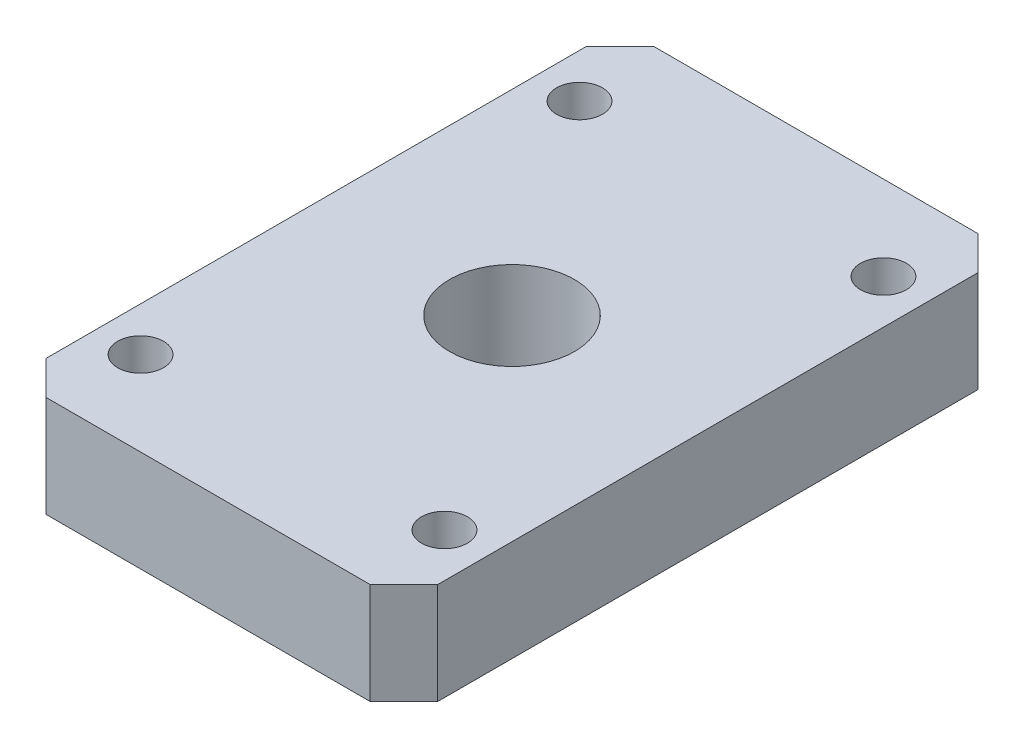
SolidWorks part; units mm, degrees
ref_plane "前视基准面" through (0, 0, 0) normal (0, 0, 1) x (1, 0, 0)
ref_plane "上视基准面" through (0, 0, 0) normal (0, 1, 0) x (1, 0, 0)
ref_plane "右视基准面" through (0, 0, 0) normal (1, 0, 0) x (0, 0, -1)
sketch "草图1" plane through (0, 0, 0) normal (0, 1, 0) x (1, 0, 0)
  line L1 (-29, 45) -> (29, 45)
  line L2 (-29, 45) -> (-29, -45)
  line L3 (-29, -45) -> (29, -45)
  line L4 (29, 45) -> (29, -45)
  line L5 (-29, 45) -> (29, -45) construction
  line L6 (-29, -45) -> (29, 45) construction
  point P0 (0, 0)
  dimension "D1" = 58
  dimension "D2" = 90
extrude "凸台-拉伸1" add sketch "草图1" along normal mid plane 15
hole_wizard "M8 螺纹孔1" positions "草图3" profile "草图2" tap size "M8" standard "ISO"
sketch "草图3" plane through (0, -7.5, 0) normal (0, 1, 0) x (1, 0, 0)
  line L0 (0, 0) -> (44.1668, 0) construction
  point P0 (-22.5, 32.5)
  point P2 (22.5, 32.5)
  point P16 (22.5, -32.5)
  point P17 (-22.5, -32.5)
  dimension "D1" = 32.5
  dimension "D2" = 22.5
  dimension "D3" = 45
cosmetic thread "孔螺蚊线6" parameters "D1"=16, "D2"=8
cosmetic thread "孔螺蚊线7" parameters "D1"=16, "D2"=8
cosmetic thread "孔螺蚊线8" parameters "D1"=16, "D2"=8
cosmetic thread "孔螺蚊线9" parameters "D1"=16, "D2"=8
sketch "草图2" plane through (-22.5, -7.5, -32.5) normal (1, 0, 0) x (0, 0, -1)
  line L0 (0, 0) -> (0, 21.7929)
  line L1 (0, 21.7929) -> (3.4, 19.75)
  line L2 (3.4, 19.75) -> (3.4, 0)
  line L5 (3.4, 0) -> (0, 0)
  line L10 (0, 21.7929) -> (-3.4, 19.75) construction
  line L11 (0, -6.35) -> (0, 107.95) construction
  dimension "螺纹孔钻头直径" = 6.8
  dimension "螺纹孔钻头深度" = 19.75
  dimension "导头角度" = 118
hole_wizard "M20x1.5 螺纹孔1" positions "草图5" profile "草图4" tap size "M20x1.5" standard "ISO"
sketch "草图5" plane through (0, 7.5, 0) normal (0, 1, 0) x (1, 0, 0)
  point P0 (0, 0)
cosmetic thread "孔螺蚊线5" parameters "D1"=16, "D2"=20
sketch "草图4" plane through (0, 7.5, 0) normal (1, 0, 0) x (0, 0, 1)
  line L0 (0, 0) -> (0, 50.058)
  line L1 (0, 50.058) -> (9.25, 44.5)
  line L2 (9.25, 44.5) -> (9.25, 0)
  line L5 (9.25, 0) -> (0, 0)
  line L10 (0, 50.058) -> (-9.25, 44.5) construction
  line L11 (0, -6.35) -> (0, 107.95) construction
  dimension "螺纹孔钻头直径" = 18.5
  dimension "螺纹孔钻头深度" = 44.5
  dimension "导头角度" = 118
chamfer "倒角1" distance 5 angle 45 4 edges at (29, 0, 45) (29, 0, -45) (-29, 0, -45) (-29, 0, 45)
